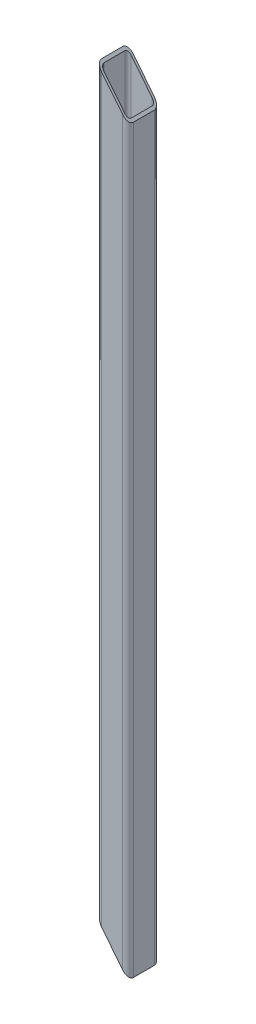
SolidWorks part; units mm, degrees
material "Q235B"
ref_plane "Front Plane" through (0, 0, 0) normal (0, 0, 1) x (1, 0, 0)
ref_plane "Top Plane" through (0, 0, 0) normal (0, 1, 0) x (1, 0, 0)
ref_plane "Right Plane" through (0, 0, 0) normal (1, 0, 0) x (0, 0, -1)
other "Configuration Table"
sketch "Sketch1" plane through (0, 0, 0) normal (0, 1, 0) x (1, 0, 0)
  line L0 (-26, -20) -> (-26, 20)
  line L1 (-20, -30) -> (20, -30)
  line L2 (-30, -20) -> (-30, 20)
  line L3 (-20, 30) -> (20, 30)
  line L4 (30, -20) -> (30, 20)
  line L5 (-30, -30) -> (30, 30) construction
  line L6 (-30, 30) -> (30, -30) construction
  line L7 (-20, 26) -> (20, 26)
  line L8 (26, -20) -> (26, 20)
  line L9 (-20, -26) -> (20, -26)
  arc A0 (20, -30) -> (30, -20) centre (20, -20) ccw
  arc A1 (-20, -30) -> (-30, -20) centre (-20, -20) cw
  arc A2 (20, 30) -> (30, 20) centre (20, 20) cw
  arc A3 (-30, 20) -> (-20, 30) centre (-20, 20) cw
  arc A4 (-26, 20) -> (-20, 26) centre (-20, 20) cw
  arc A5 (20, 26) -> (26, 20) centre (20, 20) cw
  arc A6 (20, -26) -> (26, -20) centre (20, -20) ccw
  arc A7 (-20, -26) -> (-26, -20) centre (-20, -20) cw
  point P0 (0, 0)
  dimension "D2" = 10
  dimension "D1" = 60
  dimension "D3" = 4
extrude "Boss-Extrude1" add sketch "Sketch1" along normal blind 2000
sketch "Sketch2" plane through (0, 0, 30) normal (0, 0, 1) x (1, 0, 0)
  line L0 (30, 0) -> (-30, 75.0273)
  line L1 (-30, 75.0273) -> (-170.2437, -210.0076)
  line L2 (-170.2437, -210.0076) -> (30, 0)
  line L3 (-30, 2000) -> (-30, 0) construction
  line L4 (-30, 1484.0273) -> (30, 1409)
  line L5 (30, 2000) -> (30, 0) construction
  line L6 (30, 1409) -> (525.9921, 1638.5562)
  line L7 (525.9921, 1638.5562) -> (8.9776, 2080.6264)
  line L8 (8.9776, 2080.6264) -> (-421.0153, 1818.3626)
  line L9 (-421.0153, 1818.3626) -> (-30, 1484.0273)
  dimension "D1" = 880
  dimension "D3" = 1409
extrude "Cut-Extrude1" cut sketch "Sketch2" against normal through all both and the other way through all
